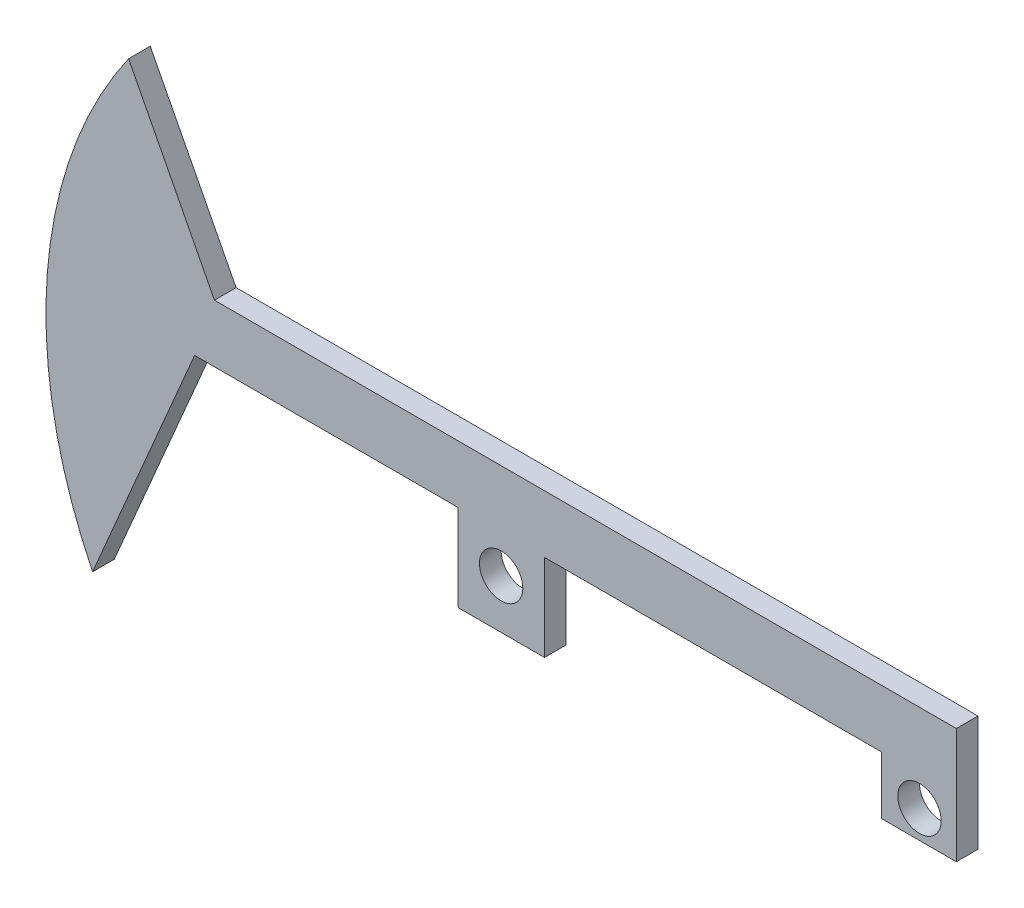
from build123d import *

# Parameters (mm, degrees)
BOSS_EXTRUDE1_DEPTH = 100
SKETCH2_R           = 100
CUT_EXTRUDE1_DEPTH  = 100


with BuildPart() as part:
    # Sketch1 → Boss-Extrude1 (new body)
    with BuildSketch(Plane.XY):
        with BuildLine():
            Line((-1718.674871456, 1206.713174795), (-1322.571209422, 440.16664507))
            Line((-1322.571209422, 440.16664507), (2100, 440.16664507))
            Line((2100, 440.16664507), (2100, 173.883799956))
            Line((2100, 173.883799956), (2100, -92.399045159))
            Line((2100, -92.399045159), (1753.894853504, -92.399045159))
            Line((1753.894853504, -92.399045159), (1753.894853504, 173.883799956))
            Line((1753.894853504, 173.883799956), (1098.892043301, 173.883799956))
            Line((1098.892043301, 173.883799956), (200, 173.883799956))
            Line((200, 173.883799956), (200, -226.116200044))
            Line((200, -226.116200044), (-200, -226.116200044))
            Line((-200, -226.116200044), (-200, 173.883799956))
            Line((-200, 173.883799956), (-1413.952786652, 173.883799956))
            Line((-1413.952786652, 173.883799956), (-1884.737570564, -926.155651122))
            ThreePointArc((-1884.737570564, -926.155651122), (-2093.663694094, 163.010232903), (-1718.674871456, 1206.713174795))
        make_face()
    extrude(amount=BOSS_EXTRUDE1_DEPTH)

    # Sketch2 → Cut-Extrude1 (cut)
    with BuildSketch(Plane.XY.offset(100)):
        with Locations((1930.037615803, 35.754280486)):
            Circle(SKETCH2_R)
        Circle(SKETCH2_R)
    extrude(amount=-CUT_EXTRUDE1_DEPTH, mode=Mode.SUBTRACT)


solid = part.part
